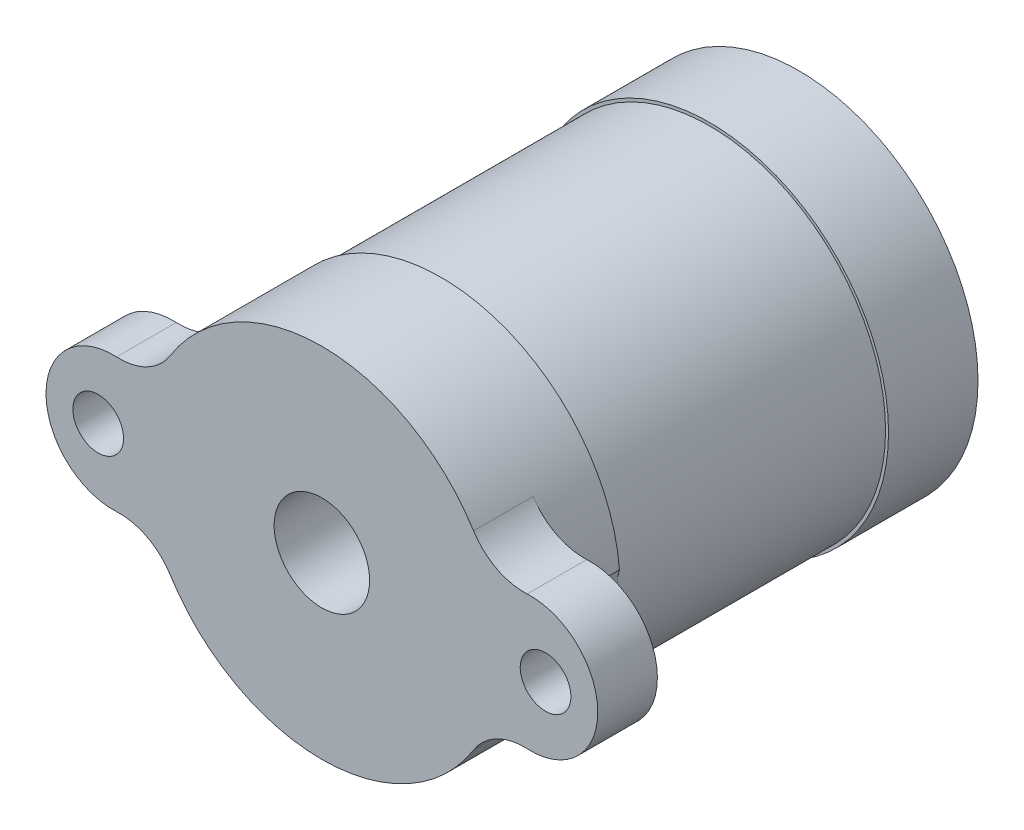
from build123d import *

# Parameters (mm, degrees)
SKETCH1_R           = 30
BOSS_EXTRUDE1_DEPTH = 20
SKETCH2_R           = 29.5
BOSS_EXTRUDE2_DEPTH = 45
SKETCH3_R           = 30
BOSS_EXTRUDE3_DEPTH = 15
SKETCH4_R           = 8
CUT_EXTRUDE1_DEPTH  = 65
SKETCH5_R           = 11.25
BOSS_EXTRUDE4_DEPTH = 10
FILLET1_R           = 10
SKETCH6_R           = 4.25
CUT_EXTRUDE2_DEPTH  = 90.101417022
SKETCH_7_2_R        = 8
CUT_EXTRUDE3_DEPTH  = 1
CUT_EXTRUDE4_REACH  = 91.101
SKETCH_7_2_2_R      = 8


with BuildPart() as part:
    # Sketch1 → Boss-Extrude1 (new body)
    with BuildSketch(Plane.XY):
        Circle(SKETCH1_R)
    extrude(amount=-BOSS_EXTRUDE1_DEPTH)

    # Sketch2 → Boss-Extrude2 (add)
    with BuildSketch(Plane(origin=(0, 0, -20), x_dir=(-1, 0, 0), z_dir=(0, 0, -1))):
        with Locations(Location((0, 0, 0), (0, 0, 180))):
            Circle(SKETCH2_R)
    extrude(amount=BOSS_EXTRUDE2_DEPTH)

    # Sketch3 → Boss-Extrude3 (add)
    with BuildSketch(Plane(origin=(0, 0, -65), x_dir=(-1, 0, 0), z_dir=(0, 0, -1))):
        with Locations(Location((0, 0, 0), (0, 0, 180))):
            Circle(SKETCH3_R)
    extrude(amount=BOSS_EXTRUDE3_DEPTH)

    # Sketch4 → Cut-Extrude1 (cut)
    with BuildSketch(Plane.XY):
        Circle(SKETCH4_R)
    extrude(amount=-CUT_EXTRUDE1_DEPTH, mode=Mode.SUBTRACT)

    # Sketch5 → Boss-Extrude4 (add)
    with BuildSketch(Plane.XY):
        with Locations((35, 0)):
            Circle(SKETCH5_R)
        with Locations((-35, 0)):
            Circle(SKETCH5_R)
    extrude(amount=-BOSS_EXTRUDE4_DEPTH)

    # Fillet1
    fillet1_edges = [part.edges().sort_by_distance(p)[0] for p in [
        (28.549107143, 9.216750042, -5),
        (28.549107143, -9.216750042, -5),
        (-28.549107143, -9.216750042, -5),
        (-28.549107143, 9.216750042, -5),
    ]]
    fillet(fillet1_edges, radius=FILLET1_R)

    # Sketch6 → Cut-Extrude2 (cut, through all)
    with BuildSketch(Plane(origin=(0, 0, -10), x_dir=(-1, 0, 0), z_dir=(0, 0, -1))):
        with Locations((37.5, 0)):
            Circle(SKETCH6_R)
        with Locations((-37.5, 0)):
            Circle(SKETCH6_R)
    extrude(amount=-CUT_EXTRUDE2_DEPTH, mode=Mode.SUBTRACT)

    # Sketch 7_2 → Cut-Extrude3 (cut)
    with BuildSketch(Plane(origin=(0, 0, -10), x_dir=(-1, 0, 0), z_dir=(0, 0, -1))):
        with Locations((37.5, 0)):
            Circle(SKETCH_7_2_R)
        with Locations((-37.5, 0)):
            Circle(SKETCH_7_2_R)
    extrude(amount=-CUT_EXTRUDE3_DEPTH, mode=Mode.SUBTRACT)

    # Sketch 7_2 2 → Cut-Extrude4 (cut, up to next)
    with BuildSketch(Plane(origin=(0, 0, -10), x_dir=(-1, 0, 0), z_dir=(0, 0, -1)), mode=Mode.PRIVATE) as cut_extrude4_sk1:
        with Locations((37.5, 0)):
            Circle(SKETCH_7_2_2_R)
    cut_extrude4_tool1 = extrude(cut_extrude4_sk1.sketch, amount=CUT_EXTRUDE4_REACH, mode=Mode.PRIVATE) & part.part
    # Sketch 7_2 2 → Cut-Extrude4 (cut, up to next)
    with BuildSketch(Plane(origin=(0, 0, -10), x_dir=(-1, 0, 0), z_dir=(0, 0, -1)), mode=Mode.PRIVATE) as cut_extrude4_sk2:
        with Locations((-37.5, 0)):
            Circle(SKETCH_7_2_2_R)
    cut_extrude4_tool2 = extrude(cut_extrude4_sk2.sketch, amount=CUT_EXTRUDE4_REACH, mode=Mode.PRIVATE) & part.part
    add(cut_extrude4_tool1.solids().sort_by_distance((-37.5, 0, -10))[0], mode=Mode.SUBTRACT)
    add(cut_extrude4_tool2.solids().sort_by_distance((37.5, 0, -10))[0], mode=Mode.SUBTRACT)


solid = part.part
